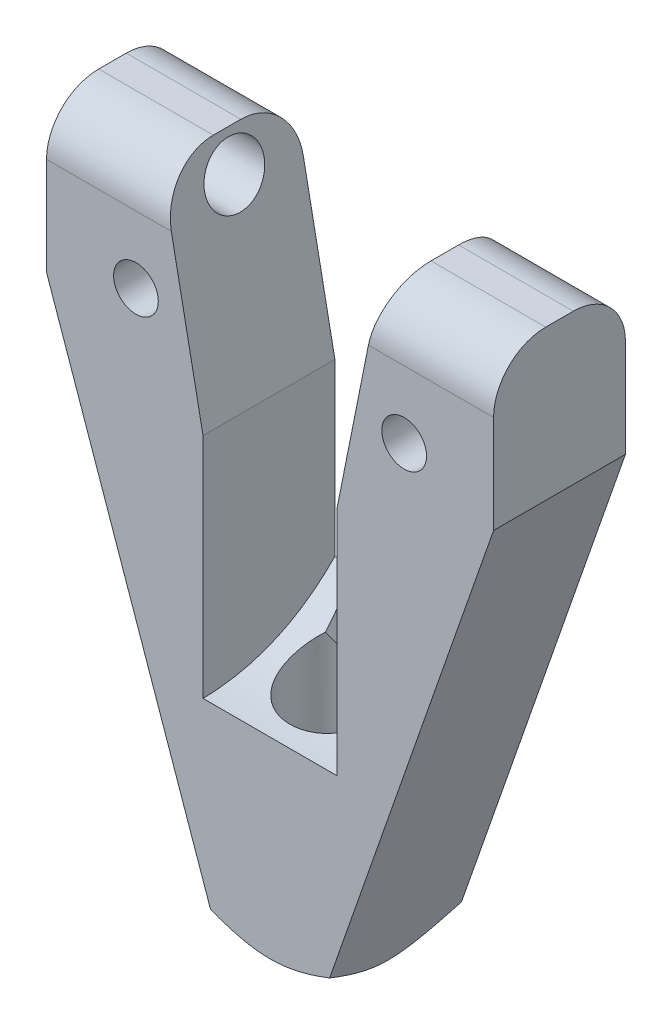
from build123d import *

# Parameters (mm, degrees)
SKETCH1_R                      = 3
BOSS_EXTRUDE2_DEPTH            = 17.7
CUT_EXTRUDE1_REACH             = 94.786
CUT_EXTRUDE1_DIRECTION_2_REACH = 94.786
SKETCH6_RX                     = 12.258033
SKETCH6_RY                     = 6.491927
CUT_EXTRUDE2_DEPTH             = 48.7
SKETCH7_R                      = 6.19409
CUT_EXTRUDE3_DEPTH             = 60.7
SKETCH8_R                      = 4
CUT_EXTRUDE4_DEPTH             = 48
FILLET1_R                      = 7
SKETCH10_OUTSIDE_W             = 249.546
SKETCH10_OUTSIDE_H             = 207.246
SKETCH10_OUTSIDE_R             = 7
CUT_EXTRUDE5_DEPTH             = 48
CUT_EXTRUDE5_TAPER             = 60


with BuildPart() as part:
    # Sketch1 → Boss-Extrude2 (new body)
    with BuildSketch(Plane.XY):
        with BuildLine():
            Line((39, -51.503555), (34.837666, -51.503555))
            Line((34.837666, -51.503555), (25.162334, -51.503555))
            Line((25.162334, -51.503555), (21, -51.503555))
            Line((21, -51.503555), (21, -28.6))
            Line((21, -28.6), (15.376404, 0))
            Line((15.376404, 0), (0, 0))
            Line((0, 0), (0, -20.136364))
            Line((0, -20.136364), (21.048788, -80.412439))
            add(Edge.make_bspline(
                [(21.669142, -82.188906), (21.466678, -81.609123), (21.259066, -81.014599), (21.048788, -80.412439)],
                knots=[0.75, 0.75, 0.75, 0.75, 1, 1, 1, 1], degree=3))
            add(Edge.make_bspline(
                [(22.255532, -83.868113), (22.06924, -83.334643), (21.871606, -82.768689), (21.669142, -82.188906)],
                knots=[0.5, 0.5, 0.5, 0.5, 0.75, 0.75, 0.75, 0.75], degree=3))
            add(Edge.make_bspline(
                [(22.524034, -84.637007), (22.439154, -84.393941), (22.348677, -84.134848), (22.255532, -83.868113)],
                knots=[0.375, 0.375, 0.375, 0.375, 0.5, 0.5, 0.5, 0.5], degree=3))
            add(Edge.make_bspline(
                [(22.758263, -85.307753), (22.688292, -85.107381), (22.608914, -84.880073), (22.524034, -84.637007)],
                knots=[0.25, 0.25, 0.25, 0.25, 0.375, 0.375, 0.375, 0.375], degree=3))
            add(Edge.make_bspline(
                [(22.855261, -85.585519), (22.825847, -85.50129), (22.793248, -85.407938), (22.758263, -85.307753)],
                knots=[0.1875, 0.1875, 0.1875, 0.1875, 0.25, 0.25, 0.25, 0.25], degree=3))
            add(Edge.make_bspline(
                [(22.932474, -85.806631), (22.910958, -85.745015), (22.884674, -85.669748), (22.855261, -85.585519)],
                knots=[0.125, 0.125, 0.125, 0.125, 0.1875, 0.1875, 0.1875, 0.1875], degree=3))
            add(Edge.make_bspline(
                [(23, -86), (22.975508, -85.929864), (22.932474, -85.806631)],
                knots=[0, 0, 0, 0.125, 0.125, 0.125], degree=2))
            Line((23, -86), (37, -86))
            add(Edge.make_bspline(
                [(37.068167, -85.804796), (37.025162, -85.927946), (37, -86)],
                knots=[0.875, 0.875, 0.875, 1, 1, 1], degree=2))
            add(Edge.make_bspline(
                [(37.242328, -85.306061), (37.171936, -85.507639), (37.111171, -85.681646), (37.068167, -85.804796)],
                knots=[0.75, 0.75, 0.75, 0.75, 0.875, 0.875, 0.875, 0.875], degree=3))
            add(Edge.make_bspline(
                [(37.47673, -84.63482), (37.392157, -84.877005), (37.31272, -85.104482), (37.242328, -85.306061)],
                knots=[0.625, 0.625, 0.625, 0.625, 0.75, 0.75, 0.75, 0.75], degree=3))
            add(Edge.make_bspline(
                [(37.744144, -83.869041), (37.651111, -84.135454), (37.561302, -84.392634), (37.47673, -84.63482)],
                knots=[0.5, 0.5, 0.5, 0.5, 0.625, 0.625, 0.625, 0.625], degree=3))
            add(Edge.make_bspline(
                [(38.330881, -82.18884), (38.128355, -82.768803), (37.930211, -83.336215), (37.744144, -83.869041)],
                knots=[0.25, 0.25, 0.25, 0.25, 0.5, 0.5, 0.5, 0.5], degree=3))
            add(Edge.make_bspline(
                [(38.951212, -80.412439), (38.741, -81.014409), (38.533408, -81.608878), (38.330881, -82.18884)],
                knots=[0, 0, 0, 0, 0.25, 0.25, 0.25, 0.25], degree=3))
            Line((38.951212, -80.412439), (60, -20.136364))
            Line((60, -20.136364), (60, 0))
            Line((60, 0), (44.6, 0))
            Line((44.6, 0), (39, -28))
            Line((39, -28), (39, -51.503555))
        make_face()
        with Locations((48, -16)):
            Circle(SKETCH1_R, mode=Mode.SUBTRACT)
        with Locations((12, -16)):
            Circle(SKETCH1_R, mode=Mode.SUBTRACT)
    extrude(amount=BOSS_EXTRUDE2_DEPTH)

    # Sketch2 → Cut-Revolve2 (revolve, cut)
    with BuildSketch(Plane.ZY.offset(-30), mode=Mode.PRIVATE) as cut_revolve2_sk:
        with BuildLine():
            ThreePointArc((11.5, -81.75), (11.729241, -80.820262), (12.364412, -80.103659))
            ThreePointArc((12.364412, -80.103659), (14.333443, -77.882187), (15.04409, -75))
            Line((15.04409, -75), (15.04409, -57.48))
            Line((15.04409, -57.48), (8.85, -57.48))
            Line((8.85, -57.48), (8.85, -86))
            Line((8.85, -86), (11.5, -86))
            Line((11.5, -86), (11.5, -81.75))
        make_face()
    revolve(cut_revolve2_sk.sketch.rotate(Axis((30, -86, 8.85), (0, 1, 0)), 180), axis=Axis((30, -86, 8.85), (0, 1, 0)), mode=Mode.SUBTRACT)

    # Cut-Extrude1: up to this face of the body (flat: up to its plane)
    cut_extrude1_end = Plane(part.part.faces().sort_by_distance((39, -39.751777, 8.85))[0])
    # Sketch3 → Cut-Extrude1 (cut, up to the picked face)
    with BuildSketch(Plane.ZY.offset(-30), mode=Mode.PRIVATE) as cut_extrude1_sk1:
        with BuildLine():
            Line((0, -51.503555), (17.7, -51.503555))
            Line((17.7, -51.503555), (17.7, -59.152297))
            add(Edge.make_bspline(
                [(17.7, -59.152297), (7.335394, -59.008853), (0, -51.503555)],
                knots=[0, 0, 0, 1, 1, 1], degree=2))
        make_face()
    cut_extrude1_tool1 = split(extrude(cut_extrude1_sk1.sketch, amount=-CUT_EXTRUDE1_REACH, mode=Mode.PRIVATE), bisect_by=cut_extrude1_end, keep=Keep.BOTH, mode=Mode.PRIVATE)
    add(cut_extrude1_tool1.solids().sort_by(Axis((30, -54.604638, 10.907898), (1, 0, 0)))[0], mode=Mode.SUBTRACT)

    # Cut-Extrude1 direction 2: up to this face of the body (flat: up to its plane)
    cut_extrude1_direction_2_end = Plane(part.part.faces().sort_by_distance((21, -40.051777, 8.85))[0])
    # Sketch3 → Cut-Extrude1 direction 2 (cut, up to the picked face)
    with BuildSketch(Plane.ZY.offset(-30), mode=Mode.PRIVATE) as cut_extrude1_direction_2_sk1:
        with BuildLine():
            Line((0, -51.503555), (17.7, -51.503555))
            Line((17.7, -51.503555), (17.7, -59.152297))
            add(Edge.make_bspline(
                [(17.7, -59.152297), (7.335394, -59.008853), (0, -51.503555)],
                knots=[0, 0, 0, 1, 1, 1], degree=2))
        make_face()
    cut_extrude1_direction_2_tool1 = split(extrude(cut_extrude1_direction_2_sk1.sketch, amount=CUT_EXTRUDE1_DIRECTION_2_REACH, mode=Mode.PRIVATE), bisect_by=cut_extrude1_direction_2_end, keep=Keep.BOTH, mode=Mode.PRIVATE)
    add(cut_extrude1_direction_2_tool1.solids().sort_by(Axis((30, -54.604638, 10.907898), (-1, 0, 0)))[0], mode=Mode.SUBTRACT)

    # Sketch6 → Cut-Extrude2 (cut)
    with BuildSketch(Plane(origin=(0, 0, 8.85), x_dir=(-1, 0, 0), z_dir=(0, 0, -1))):
        with Locations(Location((-30, -47.968312), (0, 0, 90))):
            Ellipse(SKETCH6_RX, SKETCH6_RY)
    extrude(amount=CUT_EXTRUDE2_DEPTH, mode=Mode.SUBTRACT)

    # Sketch7 → Cut-Extrude3 (cut)
    with BuildSketch(Plane(origin=(0, 0, 0), x_dir=(1, 0, 0), z_dir=(0, 1, 0))):
        with Locations(Location((30, -8.85, 0), (0, 0, 90))):
            Circle(SKETCH7_R)
    extrude(amount=-CUT_EXTRUDE3_DEPTH, mode=Mode.SUBTRACT)

    # Sketch8 → Cut-Extrude4 (cut)
    with BuildSketch(Plane.ZY.offset(-6)):
        with Locations((8.85, -5)):
            Circle(SKETCH8_R)
    extrude(amount=-CUT_EXTRUDE4_DEPTH, mode=Mode.SUBTRACT)

    # Fillet1
    fillet1_edges = [part.edges().sort_by_distance(p)[0] for p in [
        (7.688202, 0, 17.7),
        (52.3, 0, 0),
        (7.688202, 0, 0),
        (52.3, 0, 17.7),
    ]]
    fillet(fillet1_edges, radius=FILLET1_R)

    # Sketch10 outside → Cut-Extrude5 (cut)
    with BuildSketch(Plane.XZ.offset(86)):
        with Locations((30, 8.85)):
            Rectangle(SKETCH10_OUTSIDE_W, SKETCH10_OUTSIDE_H)
        with Locations((30, 8.85)):
            Circle(SKETCH10_OUTSIDE_R, mode=Mode.SUBTRACT)
    extrude(amount=-CUT_EXTRUDE5_DEPTH, taper=CUT_EXTRUDE5_TAPER, mode=Mode.SUBTRACT)


solid = part.part
